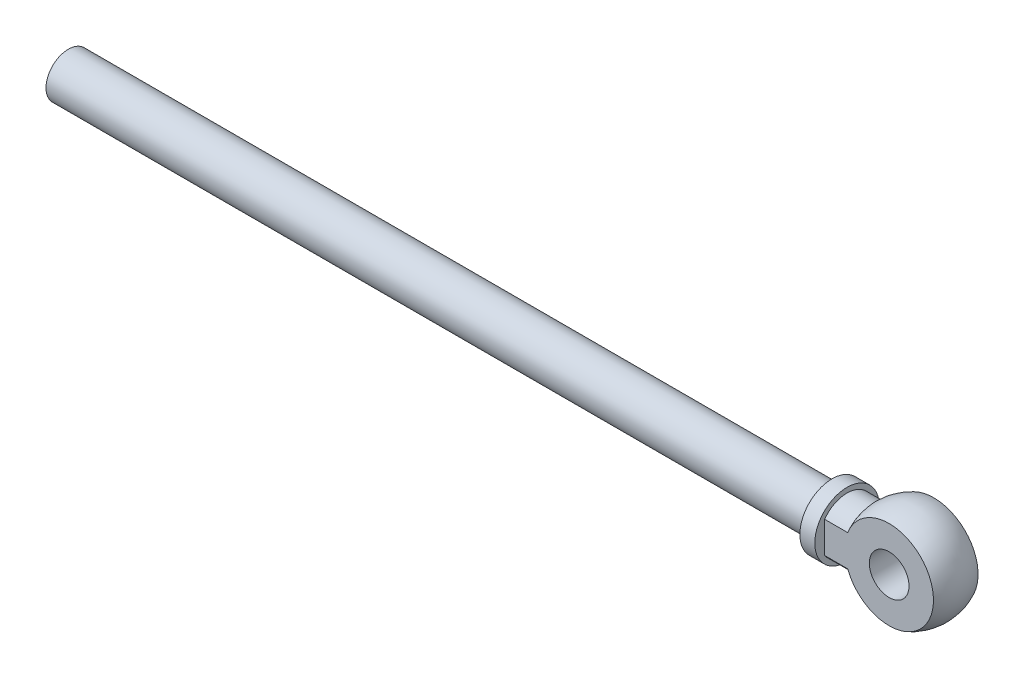
SolidWorks part; units mm, degrees
ref_plane "Front Plane" through (0, 0, 0) normal (0, 0, 1) x (1, 0, 0)
ref_plane "Top Plane" through (0, 0, 0) normal (0, 1, 0) x (1, 0, 0)
ref_plane "Right Plane" through (0, 0, 0) normal (1, 0, 0) x (0, 0, -1)
sketch "Sketch 1" plane through (0, 0, 0) normal (0, 0, 1) x (1, 0, 0)
  line L0 (0, 257.8235) -> (0, -280.0588) construction
  line L1 (-587.6471, 0) -> (491.2941, 0) construction
  line L2 (-750, 0) -> (-750, 22.5)
  line L3 (-750, 22.5) -> (20, 22.5)
  line L4 (20, 22.5) -> (20, 32.5)
  line L5 (20, 32.5) -> (35, 32.5)
  line L6 (35, 32.5) -> (35, 27.5)
  line L7 (35, 27.5) -> (58.2418, 27.5)
  line L8 (-750, 0) -> (150, 0)
  arc A0 (150, 0) -> (58.2418, 27.5) centre (100, 0) ccw
  dimension "D7" = 100
  dimension "D8" = 50
  dimension "D1" = 750
  dimension "D2" = 45
  dimension "D3" = 20
  dimension "D4" = 10
  dimension "D5" = 5
  dimension "D6" = 15
revolve "Revolve 1" add sketch "Sketch 1" angle 360 about L8
sketch "Sketch 2" plane through (35, 0, 0) normal (1, 0, 0) x (0, 0, -1)
  line L0 (0, 79.4836) -> (0, -75.1416) construction
  line L1 (-96.7312, 0) -> (103.7267, 0) construction
  line L2 (22.5, 68.3873) -> (22.5, -68.3873)
  line L3 (-59.4074, 68.3873) -> (-22.5, 68.3873)
  line L4 (-59.4074, 68.3873) -> (-59.4074, -68.3873)
  line L5 (-59.4074, -68.3873) -> (-22.5, -68.3873)
  line L6 (-22.5, 68.3873) -> (-22.5, -68.3873)
  line L7 (59.4074, -68.3873) -> (22.5, -68.3873)
  line L8 (59.4074, 68.3873) -> (59.4074, -68.3873)
  line L9 (59.4074, 68.3873) -> (22.5, 68.3873)
  dimension "D1" = 45
  dimension "D2" = 36.9074
  dimension "D3" = 136.7746
extrude "Cut-Extrude 1" cut sketch "Sketch 2" along normal through all
sketch "Sketch 3" plane through (0, 0, -22.5) normal (0, 0, -1) x (-1, 0, 0)
  circle A0 centre (-100, 0) radius 20
  dimension "D1" = 40
extrude "Cut-Extrude 2" cut sketch "Sketch 3" against normal through all
